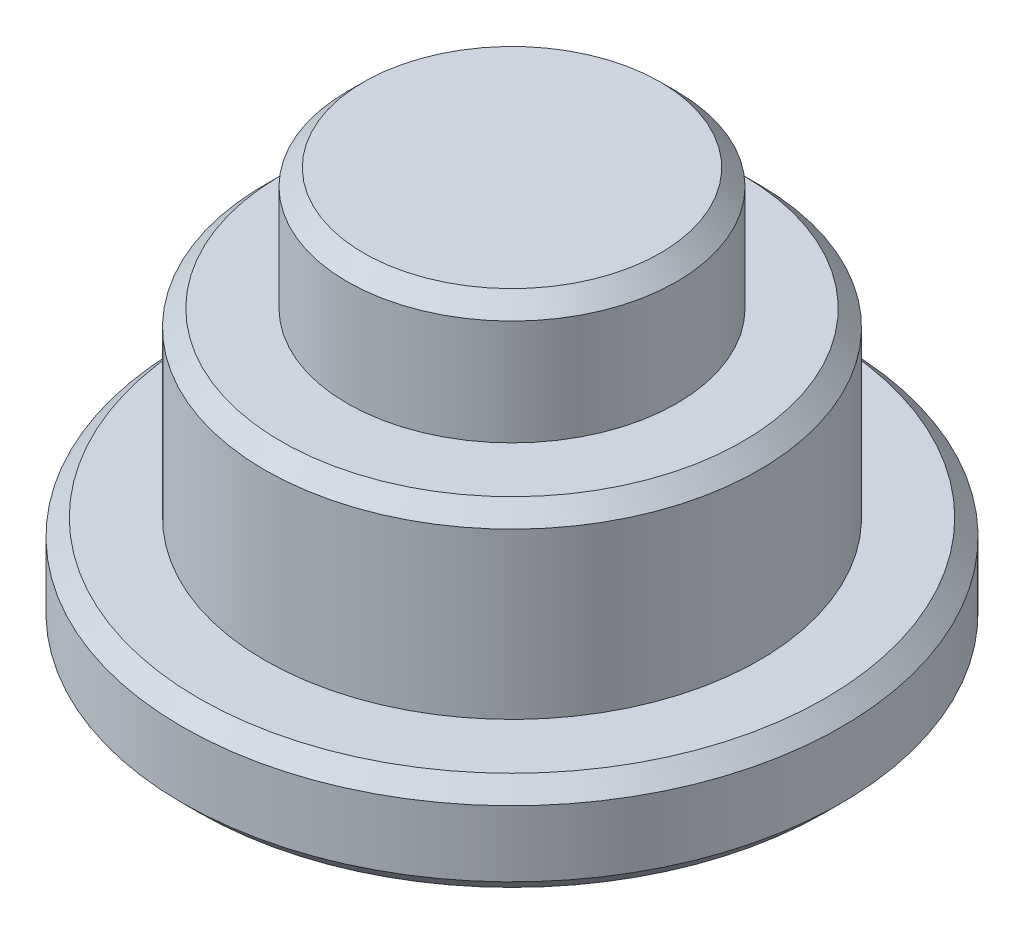
SolidWorks part; units mm, degrees
material "Q235B"
ref_plane "Front Plane" through (0, 0, 0) normal (0, 0, 1) x (1, 0, 0)
ref_plane "Top Plane" through (0, 0, 0) normal (0, 1, 0) x (1, 0, 0)
ref_plane "Right Plane" through (0, 0, 0) normal (1, 0, 0) x (0, 0, -1)
sketch "Sketch1" plane through (0, 0, 0) normal (0, 0, 1) x (1, 0, 0)
  line L0 (131.6628, -334.304) -> (131.6628, -338.004)
  line L1 (131.6628, -338.004) -> (129.1628, -338.004)
  line L2 (129.1628, -337.504) -> (129.1628, -343.504) construction
  line L3 (129.1628, -338.004) -> (129.1628, -343.504)
  line L4 (129.1628, -343.504) -> (126.6628, -343.504)
  line L5 (179.1628, -343.504) -> (-190.8372, -343.504) construction
  line L6 (126.6628, -343.504) -> (126.6628, -346.504)
  line L7 (126.6628, -346.504) -> (136.6628, -346.504)
  line L8 (136.6628, -346.504) -> (136.6628, -334.304) construction
  line L9 (124.1628, -334.304) -> (144.6628, -334.304) construction
  line L10 (136.6628, -334.304) -> (131.6628, -334.304)
  line L11 (136.6628, -334.304) -> (136.6628, -346.504)
  dimension "D1" = 7.5
  dimension "D2" = 5.5
  dimension "D3" = 3
  dimension "D4" = 20
revolve "Revolve1" add sketch "Sketch1" angle 360 about L8
chamfer "Chamfer1" distance 0.5 angle 45 4 edges at (136.6628, -346.504, -10) (136.6628, -343.504, -10) (136.6628, -338.004, -7.5) (136.6628, -334.304, -5)
